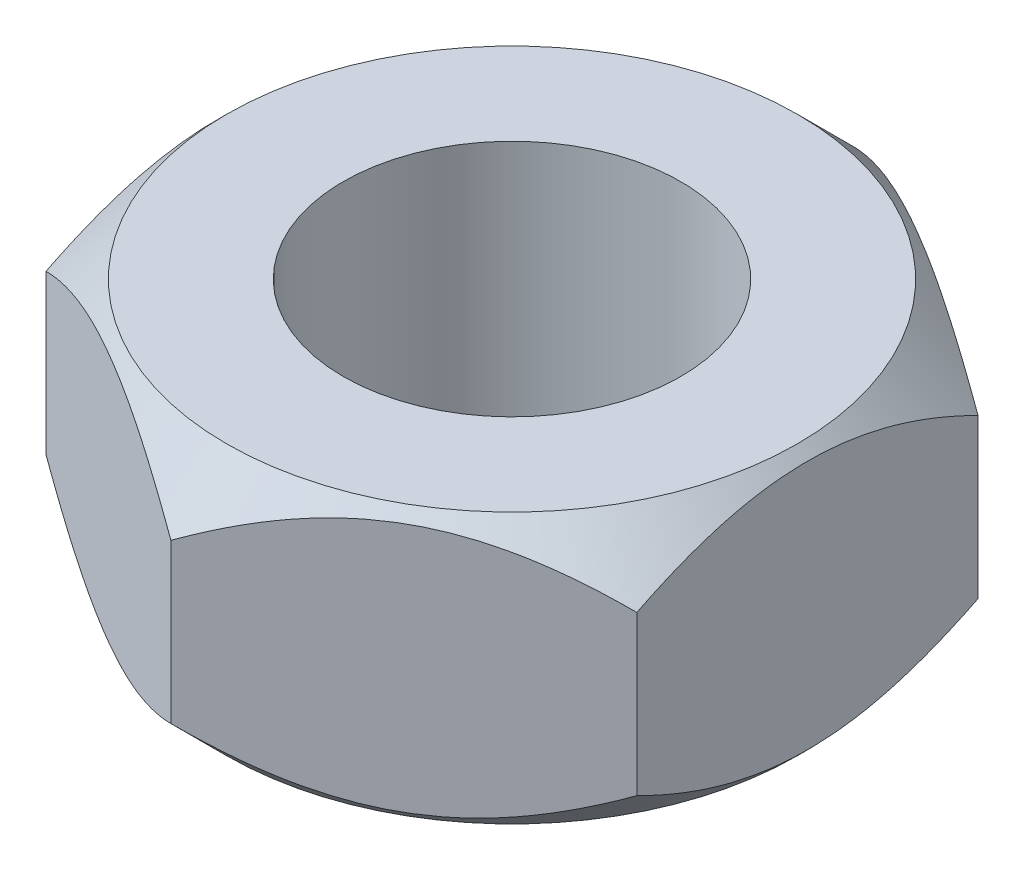
SolidWorks part; units mm, degrees
material "AISI 304"
ref_plane "Front Plane" through (0, 0, 0) normal (0, 0, 1) x (1, 0, 0)
ref_plane "Top Plane" through (0, 0, 0) normal (0, 1, 0) x (1, 0, 0)
ref_plane "Right Plane" through (0, 0, 0) normal (1, 0, 0) x (0, 0, -1)
sketch "Sketch1" plane through (0, 0, 0) normal (0, 1, 0) x (1, 0, 0)
  line L0 (-3.4644, 0) -> (4.0384, 0) construction
  line L2 (0, 4.0415) -> (-3.5, 2.0207)
  line L3 (-3.5, 2.0207) -> (-3.5, -2.0207)
  line L4 (-3.5, -2.0207) -> (0, -4.0415)
  line L5 (0, -4.0415) -> (3.5, -2.0207)
  line L6 (3.5, -2.0207) -> (3.5, 2.0207)
  line L7 (3.5, 2.0207) -> (0, 4.0415)
  circle A0 centre (0, 0) radius 3.5 construction
  dimension "D1" = 7
extrude "Boss-Extrude1" add sketch "Sketch1" along normal blind 3.2
ref_plane "Plane1" through (0, 0, 0) normal (-0.5, 0, 0.866) x (0.866, 0, 0.5)
ref_plane "Plane2" through (0, 1.6, 0) normal (0, 1, 0) x (1, 0, 0)
sketch "Sketch3" plane through (0, 0, 0) normal (-0.5, 0, 0.866) x (0.866, 0, 0.5)
  line L0 (4.0415, 3.2) -> (4.0415, 2.54)
  line L1 (4.0415, 3.2) -> (4.0415, 0) construction
  line L2 (4.0415, 3.2) -> (3.3815, 3.2)
  line L3 (3.3815, 3.2) -> (4.0415, 2.54)
  line L4 (2.943, 1.6) -> (-2.943, 1.6) construction
  line L5 (4.0415, 0) -> (4.0415, 0.66)
  line L6 (4.0415, 0) -> (3.3815, 0)
  line L7 (3.3815, 0) -> (4.0415, 0.66)
  dimension "D2" = 0.66
sketch "Sketch6" plane through (0, 0, 0) normal (-0.5, 0, 0.866) x (0.866, 0, 0.5)
  line L0 (0, -1.0158) -> (0, 3.489) construction
revolve "Cut-Revolve2" cut sketch "Sketch3" angle 360 about L0
sketch "Sketch8" plane through (0, 3.2, 0) normal (0, 1, 0) x (1, 0, 0)
  circle A0 centre (0, 0) radius 2
  dimension "D1" = 4
extrude "Cut-Extrude1" cut sketch "Sketch8" against normal through all
cosmetic thread "Cosmetic Thread1" parameters "D2"=4
